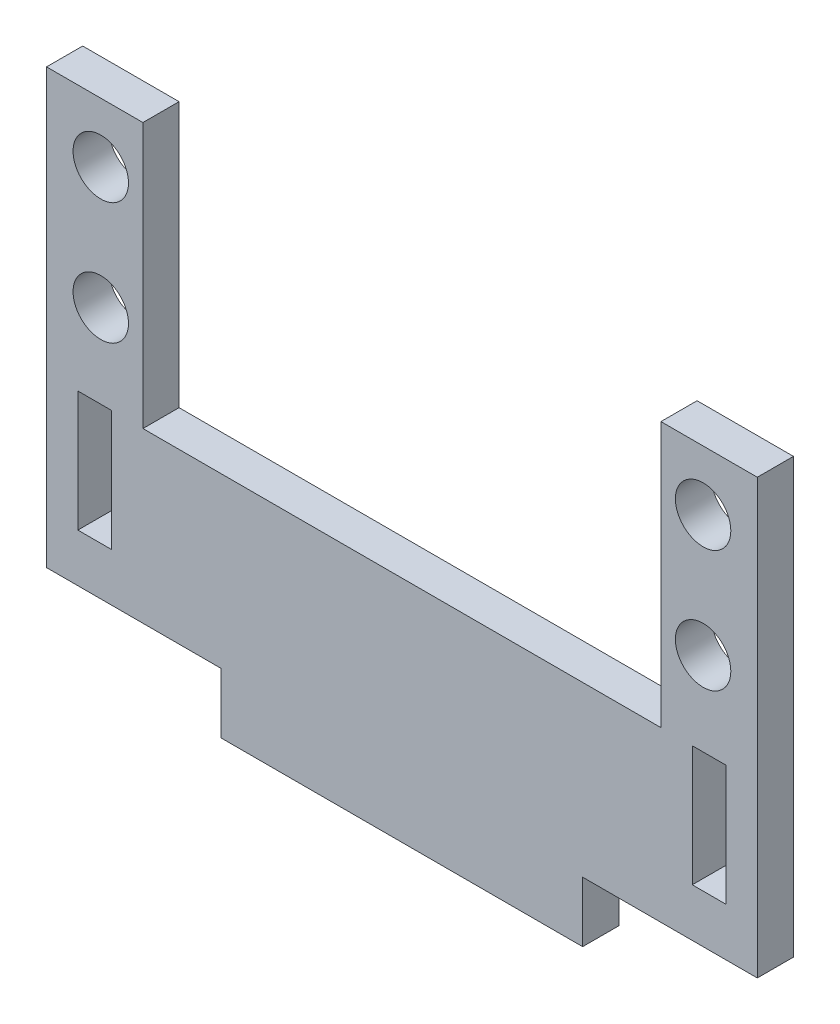
from build123d import *

# Parameters (mm, degrees)
SKETCH1_R           = 2.3
BOSS_EXTRUDE1_DEPTH = 3
SKETCH3_W           = 2.8
SKETCH3_H           = 10
CUT_EXTRUDE1_DEPTH  = 10
SKETCH4_W           = 30
SKETCH4_H           = 3
BOSS_EXTRUDE2_DEPTH = 5


with BuildPart() as part:
    # Sketch1 → Boss-Extrude1 (new body)
    with BuildSketch(Plane.XY):
        Polygon((0, 0), (8, 0), (8, -22), (51, -22), (51, 0), (59, 0), (59, -36), (0, -36), align=None)
        with Locations((4.5, -15.05)):
            Circle(SKETCH1_R, mode=Mode.SUBTRACT)
        with Locations((4.5, -4.95)):
            Circle(SKETCH1_R, mode=Mode.SUBTRACT)
        with Locations((54.5, -4.95)):
            Circle(SKETCH1_R, mode=Mode.SUBTRACT)
        with Locations((54.5, -15.05)):
            Circle(SKETCH1_R, mode=Mode.SUBTRACT)
    extrude(amount=BOSS_EXTRUDE1_DEPTH)

    # Sketch3 → Cut-Extrude1 (cut)
    with BuildSketch(Plane.XY.offset(3)):
        with Locations((4, -27)):
            Rectangle(SKETCH3_W, SKETCH3_H)
        with Locations((55, -27)):
            Rectangle(SKETCH3_W, SKETCH3_H)
    extrude(amount=-CUT_EXTRUDE1_DEPTH, mode=Mode.SUBTRACT)

    # Sketch4 → Boss-Extrude2 (add)
    with BuildSketch(Plane.XZ.offset(36)):
        with Locations((29.5, 1.5)):
            Rectangle(SKETCH4_W, SKETCH4_H)
    extrude(amount=BOSS_EXTRUDE2_DEPTH)


solid = part.part
